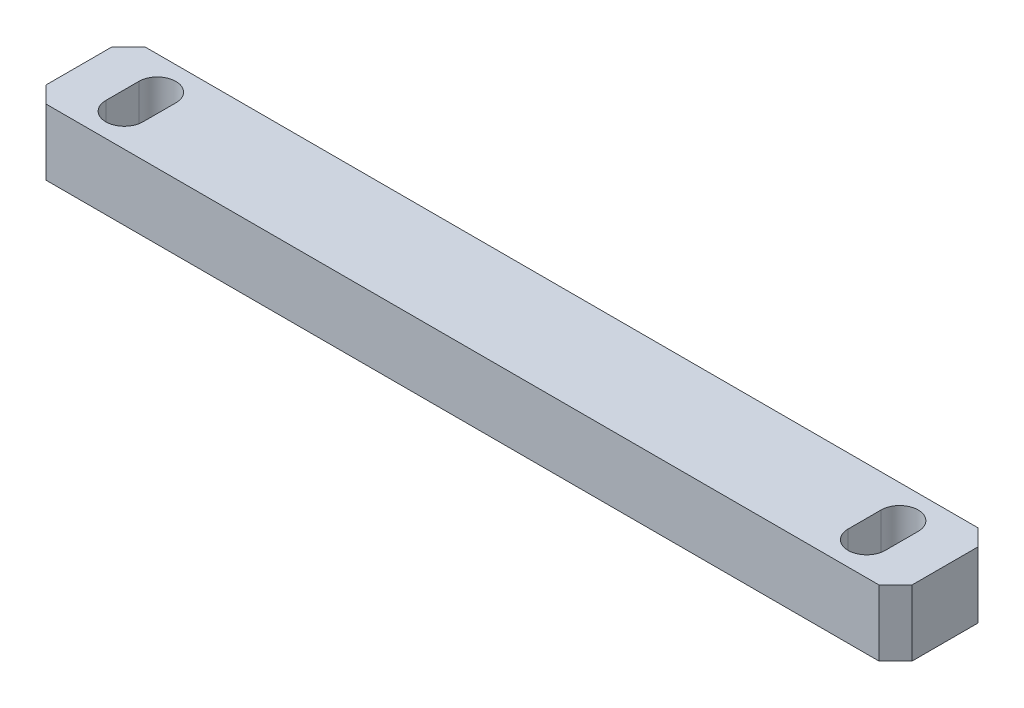
from build123d import *

# Parameters (mm, degrees)
SKETCH1_W           = 105
SKETCH1_H           = 12
BOSS_EXTRUDE1_DEPTH = 8
CHAMFER1_SIZE       = 2
SKETCH2_R           = 2.25
CUT_EXTRUDE1_DEPTH  = 10
CUT_EXTRUDE2_DEPTH  = 10


with BuildPart() as part:
    # Sketch1 → Boss-Extrude1 (new body)
    with BuildSketch(Plane(origin=(0, 0, 0), x_dir=(1, 0, 0), z_dir=(0, 1, 0))):
        with Locations((52.5, 6)):
            Rectangle(SKETCH1_W, SKETCH1_H)
    extrude(amount=BOSS_EXTRUDE1_DEPTH)

    # Chamfer1
    chamfer1_edges = [part.edges().sort_by_distance(p)[0] for p in [
        (0, 4, -12),
        (105, 4, -12),
        (105, 4, 0),
        (0, 4, 0),
    ]]
    chamfer(chamfer1_edges, length=CHAMFER1_SIZE)

    # Sketch2 → Cut-Extrude1 (cut)
    with BuildSketch(Plane(origin=(0, 8, 0), x_dir=(1, 0, 0), z_dir=(0, 1, 0))):
        with Locations(Location((7.5, 6, 0), (0, 0, 270))):
            Circle(SKETCH2_R)
        with Locations(Location((97.5, 6, 0), (0, 0, 90))):
            Circle(SKETCH2_R)
    extrude(amount=-CUT_EXTRUDE1_DEPTH, mode=Mode.SUBTRACT)

    # Sketch3 → Cut-Extrude2 (cut)
    with BuildSketch(Plane(origin=(0, 8, 0), x_dir=(1, 0, 0), z_dir=(0, 1, 0))):
        with BuildLine():
            Line((5.25, 4), (5.25, 8))
            ThreePointArc((5.25, 8), (7.5, 10.25), (9.75, 8))
            Line((9.75, 8), (9.75, 4))
            ThreePointArc((9.75, 4), (7.5, 1.75), (5.25, 4))
        make_face()
        with BuildLine():
            Line((99.75, 4), (99.75, 8))
            ThreePointArc((99.75, 8), (97.5, 10.25), (95.25, 8))
            Line((95.25, 8), (95.25, 4))
            ThreePointArc((95.25, 4), (97.5, 1.75), (99.75, 4))
        make_face()
    extrude(amount=-CUT_EXTRUDE2_DEPTH, mode=Mode.SUBTRACT)


solid = part.part
